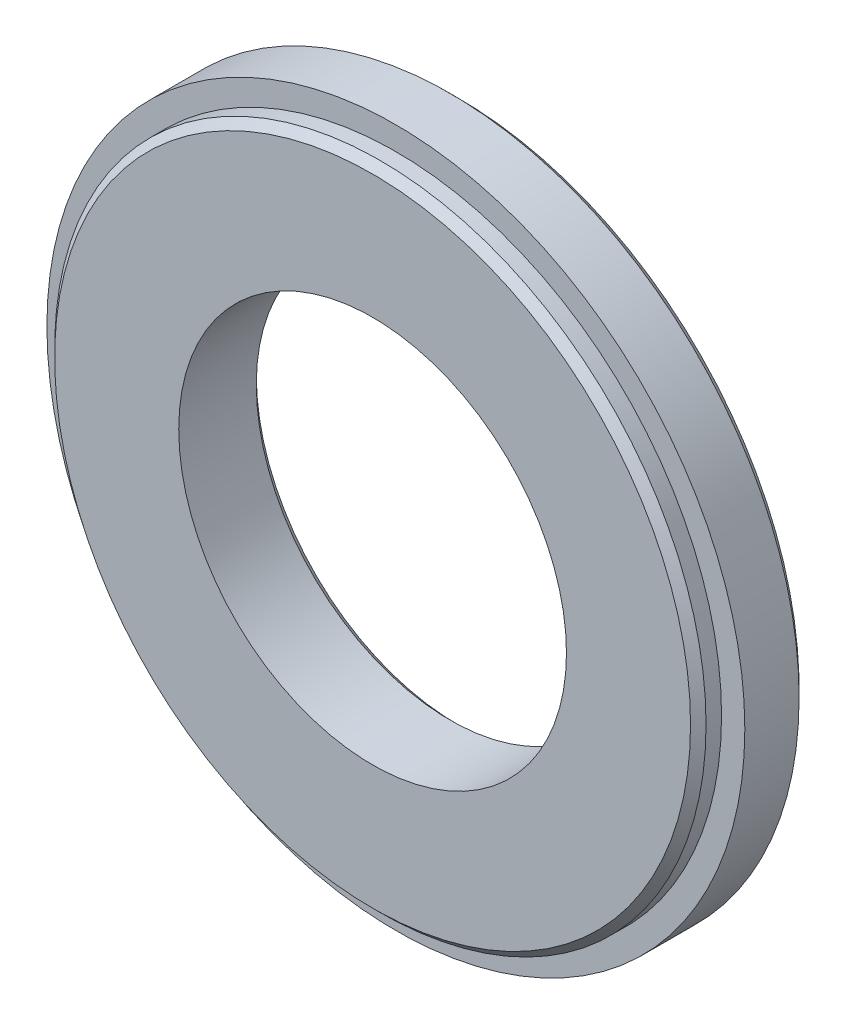
SolidWorks part; units mm, degrees
material "Q235B"
ref_plane "Front Plane" through (0, 0, 0) normal (0, 0, 1) x (1, 0, 0)
ref_plane "Top Plane" through (0, 0, 0) normal (0, 1, 0) x (1, 0, 0)
ref_plane "Right Plane" through (0, 0, 0) normal (1, 0, 0) x (0, 0, -1)
sketch "Sketch1" plane through (0, 0, 0) normal (0, 1, 0) x (1, 0, 0)
  line L0 (0, 0) -> (0, 11) construction
  line L1 (25, 0) -> (42, 0)
  line L2 (42, 0) -> (42, 3)
  line L3 (42, 3) -> (45, 3)
  line L4 (45, 3) -> (45, 11)
  line L5 (45, 11) -> (25, 11)
  line L6 (25, 11) -> (25, 0)
  dimension "D1" = 50
  dimension "D2" = 84
  dimension "D3" = 3
  dimension "D4" = 11
  dimension "D5" = 90
revolve "Revolve1" add sketch "Sketch1" angle 360 about L0
sketch "Sketch2" plane through (0, 0, -11) normal (0, 0, -1) x (-1, 0, 0)
  line L0 (0, 0) -> (0, -37) construction
  circle A0 centre (0, 0) radius 37 construction
  circle A1 centre (0, -37) radius 1.5
  circle A2 centre (-32.0429, -18.5) radius 1.5
  circle A3 centre (-32.0429, 18.5) radius 1.5
  circle A4 centre (0, 37) radius 1.5
  circle A5 centre (32.0429, 18.5) radius 1.5
  circle A6 centre (32.0429, -18.5) radius 1.5
  dimension "D1" = 74
  dimension "D2" = 3
  dimension "D3" = 6
extrude "Cut-Extrude1" cut sketch "Sketch2" against normal blind 3
hole_wizard "M4 Tapped Hole1" positions "Sketch3" profile "Sketch4" tap size "M4" standard "GB"
sketch "Sketch3" plane through (0, 0, -11) normal (0, 0, -1) x (-1, 0, 0)
  point P0 (0, -37)
  point P3 (-32.0429, -18.5)
  point P6 (-32.0429, 18.5)
  point P9 (0, 37)
  point P12 (32.0429, -18.5)
  point P15 (32.0429, 18.5)
sketch "Sketch4" plane through (0, -37, -11) normal (1, 0, 0) x (0, 1, 0)
  line L0 (0, 0) -> (0, 8.9914)
  line L1 (0, 8.9914) -> (1.65, 8)
  line L2 (1.65, 8) -> (1.65, 0)
  line L5 (1.65, 0) -> (0, 0)
  line L10 (0, 8.9914) -> (-1.65, 8) construction
  line L11 (0, -6.35) -> (0, 107.95) construction
  dimension "螺纹孔钻头直径" = 3.3
  dimension "螺纹孔钻头深度" = 8
  dimension "导头角度" = 118
cosmetic thread "Hole thread 1" parameters "D1"=6, "D2"=4
cosmetic thread "Hole thread 2" parameters "D1"=6, "D2"=4
cosmetic thread "Hole thread 3" parameters "D1"=6, "D2"=4
cosmetic thread "Hole thread 4" parameters "D1"=6, "D2"=4
cosmetic thread "Hole thread 5" parameters "D1"=6, "D2"=4
cosmetic thread "Hole thread 6" parameters "D1"=6, "D2"=4
chamfer "Chamfer1" distance 0.375 angle 45 6 edges at (-1.65, -37, -11) (30.3929, -18.5, -11) (30.3929, 18.5, -11) (-1.65, 37, -11) (-33.6929, 18.5, -11) (-33.6929, -18.5, -11)
chamfer "Chamfer2" distance 1 angle 45 3 edges at (42, 0, 0) (25, 0, -11) (45, 0, -11)
